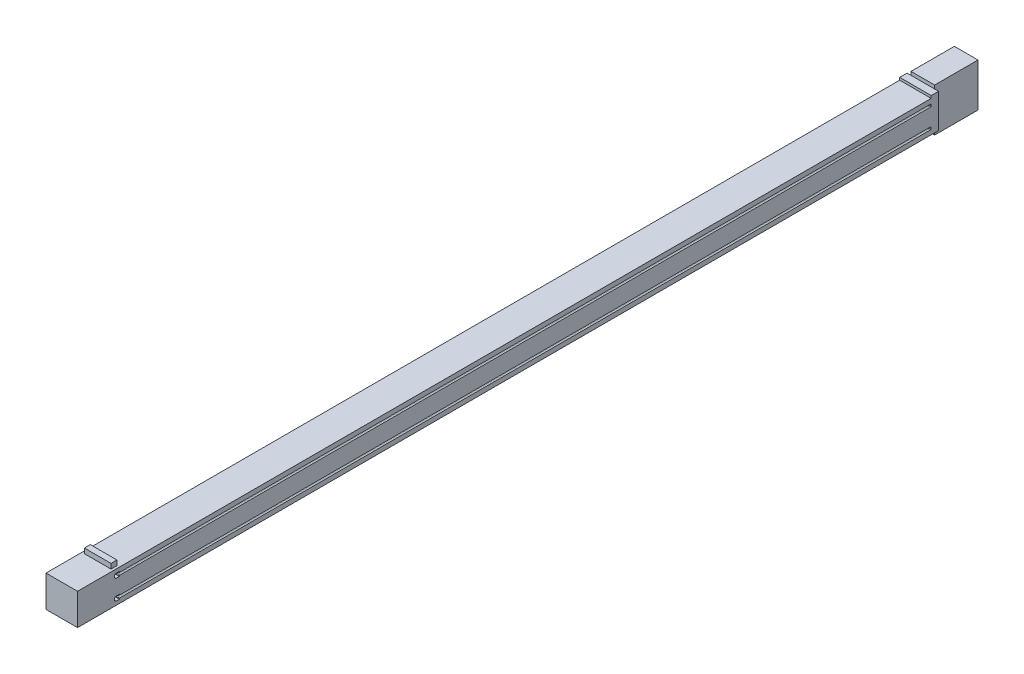
SolidWorks part; units mm, degrees
ref_plane "前视" through (0, 0, 0) normal (0, 0, 1) x (1, 0, 0)
ref_plane "上视" through (0, 0, 0) normal (0, 1, 0) x (1, 0, 0)
ref_plane "右视" through (0, 0, 0) normal (1, 0, 0) x (0, 0, -1)
sketch "草图1" plane through (0, 0, 0) normal (0, 0, 1) x (1, 0, 0)
  line L0 (41.9319, 63.6353) -> (41.9319, -24.9145) construction
  line L1 (9.9319, 6.9259) -> (9.9319, 41.9259)
  line L2 (9.9319, 56.4259) -> (73.9319, 56.4259)
  line L3 (9.9319, 46.9259) -> (12.9319, 46.9259)
  line L4 (1.2009, 24.4259) -> (59.3506, 24.4259) construction
  line L5 (12.9319, 46.9259) -> (12.9319, 48.4259)
  line L6 (12.9319, 48.4259) -> (16.9319, 48.4259)
  line L7 (16.9319, 48.4259) -> (16.9319, 40.4259)
  line L8 (16.9319, 40.4259) -> (12.9319, 40.4259)
  line L9 (12.9319, 40.4259) -> (12.9319, 41.9259)
  line L10 (12.9319, 41.9259) -> (9.9319, 41.9259)
  line L11 (9.9319, 46.9259) -> (9.9319, 56.4259)
  line L12 (9.9319, 1.9259) -> (9.9319, -7.5741)
  line L13 (12.9319, 6.9259) -> (9.9319, 6.9259)
  line L14 (12.9319, 8.4259) -> (12.9319, 6.9259)
  line L15 (16.9319, 8.4259) -> (12.9319, 8.4259)
  line L16 (16.9319, 0.4259) -> (16.9319, 8.4259)
  line L17 (12.9319, 0.4259) -> (16.9319, 0.4259)
  line L18 (12.9319, 1.9259) -> (12.9319, 0.4259)
  line L19 (9.9319, 1.9259) -> (12.9319, 1.9259)
  line L20 (9.9319, -7.5741) -> (73.9319, -7.5741)
  line L21 (73.9319, 1.9259) -> (70.9319, 1.9259)
  line L22 (70.9319, 1.9259) -> (70.9319, 0.4259)
  line L23 (70.9319, 0.4259) -> (66.9319, 0.4259)
  line L24 (66.9319, 0.4259) -> (66.9319, 8.4259)
  line L25 (66.9319, 8.4259) -> (70.9319, 8.4259)
  line L26 (70.9319, 8.4259) -> (70.9319, 6.9259)
  line L27 (70.9319, 6.9259) -> (73.9319, 6.9259)
  line L28 (73.9319, 1.9259) -> (73.9319, -7.5741)
  line L29 (73.9319, 46.9259) -> (73.9319, 56.4259)
  line L30 (70.9319, 41.9259) -> (73.9319, 41.9259)
  line L31 (70.9319, 40.4259) -> (70.9319, 41.9259)
  line L32 (66.9319, 40.4259) -> (70.9319, 40.4259)
  line L33 (66.9319, 48.4259) -> (66.9319, 40.4259)
  line L34 (70.9319, 48.4259) -> (66.9319, 48.4259)
  line L35 (70.9319, 46.9259) -> (70.9319, 48.4259)
  line L36 (73.9319, 46.9259) -> (70.9319, 46.9259)
  line L37 (73.9319, 6.9259) -> (73.9319, 41.9259)
  point P25 (9.9319, 24.4259)
  point P26 (41.9319, -7.5741)
  point P43 (41.9319, 56.4259)
  dimension "D1" = 32
  dimension "D2" = 32
  dimension "D3" = 9.5
  dimension "D4" = 8
  dimension "D5" = 5
  dimension "D6" = 3
  dimension "D7" = 4
extrude "基体-拉伸" add sketch "草图1" against normal blind 1648
sketch "草图2" plane through (0, 0, 0) normal (0, 0, 1) x (1, 0, 0)
  line L1 (73.9319, -7.5741) -> (9.9319, -7.5741)
  line L2 (73.9319, -7.5741) -> (73.9319, 56.4259)
  line L3 (73.9319, 56.4259) -> (9.9319, 56.4259)
  line L4 (9.9319, -7.5741) -> (9.9319, 56.4259)
extrude "凸台-拉伸1" add sketch "草图2" along normal blind 85
sketch "草图4" plane through (0, 56.4259, 0) normal (0, 1, 0) x (-1, 0, 0)
  line L0 (-73.9319, -1648) -> (-73.9319, 85) construction
  line L1 (-68.9319, 0) -> (-14.9319, 0)
  line L2 (-68.9319, 0) -> (-68.9319, 12)
  line L3 (-68.9319, 12) -> (-14.9319, 12)
  line L4 (-14.9319, 0) -> (-14.9319, 12)
  line L5 (-9.9319, -1648) -> (-9.9319, 85) construction
  dimension "D1" = 5
  dimension "D2" = 5
  dimension "D3" = 12
extrude "凸台-拉伸2" add sketch "草图4" along normal blind 10
sketch "草图5" plane through (73.9319, 0, 0) normal (1, 0, 0) x (0, 0, -1)
  line L0 (1648, 46.9259) -> (0, 46.9259) construction
  line L1 (0, 48.9259) -> (-6, 48.9259)
  line L2 (0, 48.9259) -> (0, 39.9259)
  line L3 (0, 39.9259) -> (-6, 39.9259)
  line L4 (-10, 44.9259) -> (-10, 43.9259)
  line L5 (0, 8.9259) -> (-6, 8.9259)
  line L6 (0, 8.9259) -> (0, -0.0741)
  line L7 (0, -0.0741) -> (-6, -0.0741)
  line L8 (-10, 4.9259) -> (-10, 3.9259)
  line L9 (1648, 41.9259) -> (0, 41.9259) construction
  line L10 (0, 41.9259) -> (0, 46.9259) construction
  line L11 (1648, 6.9259) -> (0, 6.9259) construction
  line L12 (1648, 1.9259) -> (0, 1.9259) construction
  line L13 (0, 1.9259) -> (0, 6.9259) construction
  arc A0 (-10, 43.9259) -> (-6, 39.9259) centre (-6, 43.9259) ccw
  arc A1 (-6, 48.9259) -> (-10, 44.9259) centre (-6, 44.9259) ccw
  arc A2 (-10, 4.9259) -> (-6, 8.9259) centre (-6, 4.9259) cw
  arc A3 (-10, 3.9259) -> (-6, -0.0741) centre (-6, 3.9259) ccw
  point P16 (-10, 39.9259)
  point P27 (-10, 8.9259)
  dimension "D4" = 4
  dimension "D5" = 4
  dimension "D9" = 4
  dimension "D1" = 2
  dimension "D2" = 2
  dimension "D3" = 10
  dimension "D6" = 2
  dimension "D7" = 2
  dimension "D8" = 10
extrude "切除-拉伸1" cut sketch "草图5" against normal blind 10
ref_plane "基准面4" through (41.9319, 0, 0) normal (-1, 0, 0) x (0, 0, 1)
mirror "镜向1" about plane through (41.9319, 0, 0) normal (-1, 0, 0) of "切除-拉伸1"
sketch "草图6" plane through (0, 0, -1648) normal (0, 0, -1) x (-1, 0, 0)
  line L0 (-73.9319, 56.4259) -> (-9.9319, 56.4259) construction
  line L1 (-73.9319, -7.5741) -> (-9.9319, -7.5741)
  line L2 (-73.9319, -7.5741) -> (-73.9319, 61.4259)
  line L3 (-73.9319, 61.4259) -> (-9.9319, 61.4259)
  line L4 (-9.9319, -7.5741) -> (-9.9319, 61.4259)
  dimension "D1" = 5
extrude "凸台-拉伸3" add sketch "草图6" along normal blind 15
sketch "草图7" plane through (0, 0, -1663) normal (0, 0, -1) x (-1, 0, 0)
  line L0 (-9.9319, 61.4259) -> (-73.9319, 61.4259) construction
  line L1 (-65.9319, -19.5741) -> (-17.9319, -19.5741)
  line L2 (-65.9319, -19.5741) -> (-65.9319, 68.4259)
  line L3 (-65.9319, 68.4259) -> (-17.9319, 68.4259)
  line L4 (-17.9319, -19.5741) -> (-17.9319, 68.4259)
  line L5 (-73.9319, -7.5741) -> (-9.9319, -7.5741) construction
  line L6 (-73.9319, 61.4259) -> (-73.9319, -7.5741) construction
  line L7 (-9.9319, -7.5741) -> (-9.9319, 61.4259) construction
  dimension "D1" = 7
  dimension "D2" = 12
  dimension "D3" = 8
  dimension "D4" = 8
extrude "凸台-拉伸4" add sketch "草图7" along normal blind 88
sketch "草图8" plane through (17.9319, 0, 0) normal (-1, 0, 0) x (0, 0, 1)
  line L0 (-1751, -19.5741) -> (-1663, -19.5741) construction
  line L2 (-1648, 56.4259) -> (-1648, 61.4259) construction
  circle A0 centre (-1707, 24.4259) radius 36.5
  dimension "D1" = 73
  dimension "D2" = 44
  dimension "D3" = 59
extrude "切除-拉伸2" cut sketch "草图8" against normal blind 3
sketch "草图9" plane through (20.9319, 0, 0) normal (-1, 0, 0) x (0, 0, 1)
  circle A0 centre (-1707, 24.4259) radius 8
  circle A1 centre (-1707, 24.4259) radius 36.5 construction
  dimension "D1" = 16
extrude "凸台-拉伸5" add sketch "草图9" along normal blind 19
